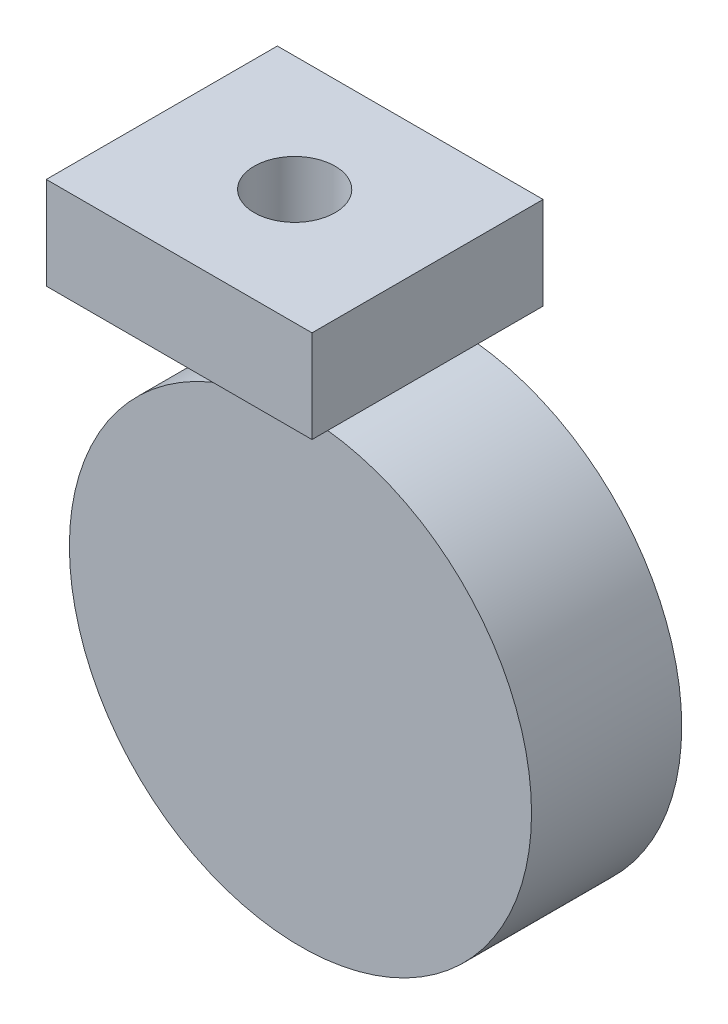
SolidWorks part; units mm, degrees
ref_plane "前视基准面" through (0, 0, 0) normal (0, 0, 1) x (1, 0, 0)
ref_plane "上视基准面" through (0, 0, 0) normal (0, 1, 0) x (1, 0, 0)
ref_plane "右视基准面" through (0, 0, 0) normal (1, 0, 0) x (0, 0, -1)
sketch "草图1" plane through (0, 0, 0) normal (0, 0, 1) x (1, 0, 0)
  circle A0 centre (0, 0) radius 100
  dimension "D1" = 200
extrude "凸台-拉伸1" add sketch "草图1" along normal mid plane 65
sketch "草图2" plane through (0, 0, 0) normal (0, 0, 1) x (1, 0, 0)
  line L0 (0, 0) -> (-35, 110) construction
  line L1 (-92.5, 150) -> (22.5, 150)
  line L2 (-92.5, 150) -> (-92.5, 110)
  line L3 (-92.5, 110) -> (22.5, 110)
  line L4 (22.5, 150) -> (22.5, 110)
  line L5 (0, 0) -> (0, 110) construction
  line L6 (-35, 110) -> (0, 110) construction
  circle A0 centre (0, 0) radius 100 construction
  point P7 (0, -100)
  dimension "D1" = 35
  dimension "D2" = 115
  dimension "D3" = 250
  dimension "D4" = 110
extrude "凸台-拉伸2" add sketch "草图2" along normal mid plane 100 separate body
sketch "草图3" plane through (0, 150, 0) normal (0, 1, 0) x (1, 0, 0)
  line L0 (22.5, 50) -> (-92.5, -50) construction
  circle A0 centre (-35, 0) radius 17.4807
extrude "切除-拉伸1" cut sketch "草图3" against normal up to next (40 mm away)
